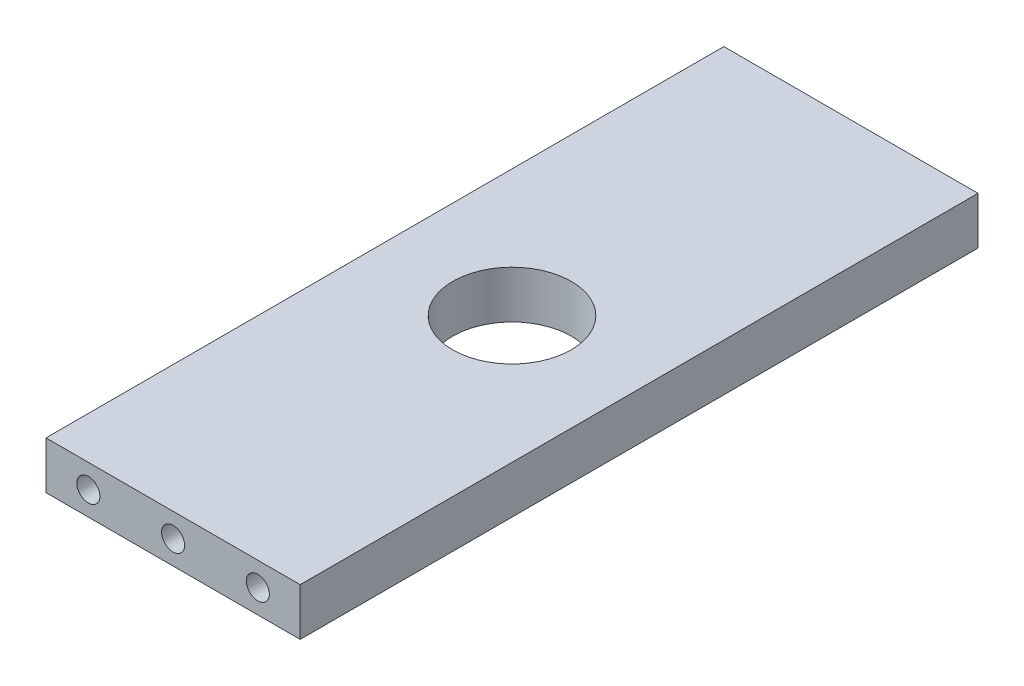
SolidWorks part; units mm, degrees
ref_plane "Front Plane" through (0, 0, 0) normal (0, 0, 1) x (1, 0, 0)
ref_plane "Top Plane" through (0, 0, 0) normal (0, 1, 0) x (1, 0, 0)
ref_plane "Right Plane" through (0, 0, 0) normal (1, 0, 0) x (0, 0, -1)
sketch "Sketch1" plane through (0, 0, 0) normal (0, 0, 1) x (1, 0, 0)
  line L0 (65.49, 334) -> (65.49, 258.2219) construction
  line L1 (27.99, 334) -> (102.99, 334)
  line L2 (27.99, 334) -> (27.99, 320)
  line L3 (27.99, 320) -> (102.99, 320)
  line L4 (102.99, 334) -> (102.99, 320)
  line L5 (56.99, 327.7975) -> (56.99, 315.7975) construction
  line L6 (56.99, 321.7975) -> (73.99, 321.7975) construction
  line L7 (73.99, 315.7975) -> (73.99, 327.7975) construction
  line L8 (65.49, 321.7975) -> (65.49, 348.7193) construction
  line L10 (110, 460) -> (0, 460) construction
  dimension "D1" = 14
  dimension "D2" = 75
  dimension "D3" = 126
extrude "Boss-Extrude1" add sketch "Sketch1" along normal up to surface (200 mm away)
sketch "Sketch2" plane through (0, 334, 0) normal (0, 1, 0) x (1, 0, 0)
  line L0 (65.49, 0) -> (65.49, -200) construction
  line L1 (102.99, 0) -> (27.99, 0) construction
  line L2 (27.99, -200) -> (102.99, -200) construction
  line L3 (27.99, -100) -> (102.99, -100) construction
  line L4 (27.99, -200) -> (27.99, 0) construction
  line L5 (102.99, -200) -> (102.99, 0) construction
  circle A0 centre (65.49, -100) radius 17.5
  dimension "D1" = 35
extrude "Cut-Extrude1" cut sketch "Sketch2" against normal through all
hole_wizard "M8 Tapped Hole2" positions "Sketch3" profile "Sketch4" tap size "M8" standard "GB"
sketch "Sketch3" plane through (0, 0, 200) normal (0, 0, 1) x (1, 0, 0)
  line L0 (27.99, 327) -> (102.99, 327) construction
  line L1 (27.99, 320) -> (27.99, 334) construction
  line L2 (102.99, 334) -> (102.99, 320) construction
  line L4 (65.49, 334) -> (65.49, 320) construction
  line L5 (27.99, 334) -> (102.99, 334) construction
  line L6 (102.99, 320) -> (27.99, 320) construction
  point P17 (65.49, 327)
  point P19 (40.49, 327)
  point P21 (90.49, 327)
  dimension "D1" = 50
sketch "Sketch4" plane through (65.49, 327, 200) normal (1, 0, 0) x (0, -1, 0)
  line L0 (0, 0) -> (0, 24.2929)
  line L1 (0, 24.2929) -> (3.4, 22.25)
  line L2 (3.4, 22.25) -> (3.4, 0)
  line L5 (3.4, 0) -> (0, 0)
  line L10 (0, 24.2929) -> (-3.4, 22.25) construction
  line L11 (0, -6.35) -> (0, 107.95) construction
  dimension "螺纹孔钻头直径" = 6.8
  dimension "螺纹孔钻头深度" = 22.25
  dimension "导头角度" = 118
cosmetic thread "Cosmetic Thread1" parameters "D1"=16, "D2"=8
cosmetic thread "Cosmetic Thread2" parameters "D1"=16, "D2"=8
cosmetic thread "Cosmetic Thread3" parameters "D1"=16, "D2"=8
hole_wizard "M8 Tapped Hole3" positions "Sketch5" profile "Sketch6" tap size "M8" standard "GB"
sketch "Sketch5" plane through (0, 0, 0) normal (0, 0, -1) x (-1, 0, 0)
  point P0 (-90.49, 327)
  point P3 (-65.49, 327)
  point P6 (-40.49, 327)
sketch "Sketch6" plane through (90.49, 327, 0) normal (1, 0, 0) x (0, 1, 0)
  line L0 (0, 0) -> (0, 24.2929)
  line L1 (0, 24.2929) -> (3.4, 22.25)
  line L2 (3.4, 22.25) -> (3.4, 0)
  line L5 (3.4, 0) -> (0, 0)
  line L10 (0, 24.2929) -> (-3.4, 22.25) construction
  line L11 (0, -6.35) -> (0, 107.95) construction
  dimension "螺纹孔钻头直径" = 6.8
  dimension "螺纹孔钻头深度" = 22.25
  dimension "导头角度" = 118
cosmetic thread "Cosmetic Thread4" parameters "D1"=16, "D2"=8
cosmetic thread "Cosmetic Thread5" parameters "D1"=16, "D2"=8
cosmetic thread "Cosmetic Thread6" parameters "D1"=16, "D2"=8
